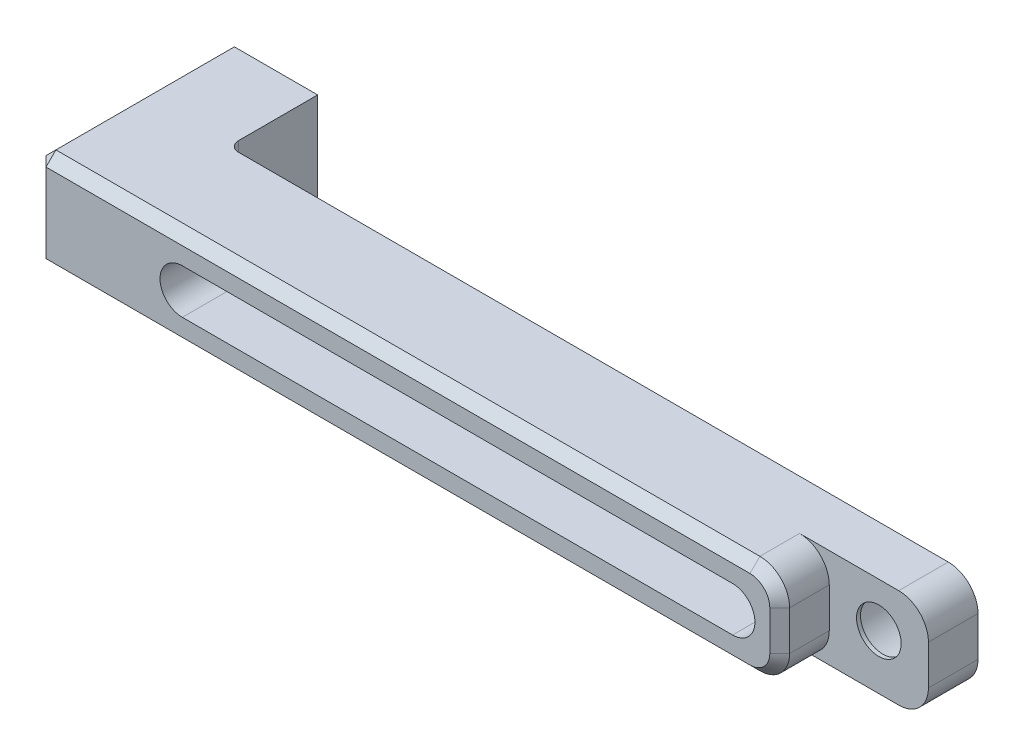
SolidWorks part; units mm, degrees
ref_plane "Front Plane" through (0, 0, 0) normal (0, 0, 1) x (1, 0, 0)
ref_plane "Top Plane" through (0, 0, 0) normal (0, 1, 0) x (1, 0, 0)
ref_plane "Right Plane" through (0, 0, 0) normal (1, 0, 0) x (0, 0, -1)
sketch "Sketch1" plane through (0, 0, 0) normal (0, 1, 0) x (1, 0, 0)
  line L1 (42.5, -5) -> (-42.5, -5)
  line L2 (42.5, -5) -> (42.5, 5)
  line L3 (42.5, 5) -> (-42.5, 5)
  line L4 (-42.5, -5) -> (-42.5, 5)
  line L5 (42.5, -5) -> (-42.5, 5) construction
  line L6 (42.5, 5) -> (-42.5, -5) construction
  point P0 (0, 0)
  dimension "D1" = 85
  dimension "D2" = 10
extrude "Boss-Extrude1" add sketch "Sketch1" along normal blind 10
sketch "Sketch2" plane through (0, 0, -5) normal (0, 0, 1) x (1, 0, 0)
  line L0 (0, 10) -> (0, 0) construction
  line L1 (-42.5, 10) -> (42.5, 10) construction
  line L2 (-27.75, 5) -> (27.75, 5) construction
  line L3 (-27.75, 9) -> (27.75, 9)
  line L4 (-27.75, 1) -> (27.75, 1)
  arc A0 (-27.75, 9) -> (-27.75, 1) centre (-27.75, 5) ccw
  arc A1 (27.75, 1) -> (27.75, 9) centre (27.75, 5) ccw
  point P7 (0, 5)
  dimension "D2" = 4
  dimension "D1" = 55.5
extrude "Cut-Extrude1" cut sketch "Sketch2" along normal blind 4.4
sketch "Sketch3" plane through (0, 0, -0.6) normal (0, 0, -1) x (-1, 0, 0)
  line L0 (-27.75, 5) -> (27.75, 5) construction
  line L1 (-27.75, 7.25) -> (27.75, 7.25)
  line L2 (-27.75, 2.75) -> (27.75, 2.75)
  line L3 (0, 0) -> (0, 10) construction
  line L4 (-42.5, 10) -> (42.5, 10) construction
  arc A0 (-27.75, 7.25) -> (-27.75, 2.75) centre (-27.75, 5) ccw
  arc A1 (27.75, 2.75) -> (27.75, 7.25) centre (27.75, 5) ccw
  point P4 (0, 5)
  dimension "D1" = 2.25
  dimension "D2" = 55.5
extrude "Cut-Extrude2" cut sketch "Sketch3" against normal through all
sketch "Sketch4" plane through (0, 0, -5) normal (0, 0, 1) x (1, 0, 0)
  line L0 (-42.5, 0) -> (42.5, 0) construction
  line L1 (-42.5, 10) -> (-33.1, 10)
  line L2 (-42.5, 10) -> (-42.5, 0)
  line L3 (-42.5, 0) -> (-33.1, 0)
  line L4 (-33.1, 10) -> (-33.1, 0)
  dimension "D1" = 9.4
extrude "Boss-Extrude2" add sketch "Sketch4" against normal blind 10 contours L4 L3 L2 L1
sketch "Sketch5" plane through (0, 0, 5) normal (0, 0, 1) x (1, 0, 0)
  line L0 (-42.5, 0) -> (42.5, 0) construction
  line L1 (42.5, 10) -> (32.5, 10)
  line L2 (42.5, 10) -> (42.5, 0)
  line L3 (42.5, 0) -> (32.5, 0)
  line L4 (32.5, 10) -> (32.5, 0)
  dimension "D1" = 10
extrude "Cut-Extrude3" cut sketch "Sketch5" against normal blind 5
sketch "Sketch6" plane through (0, 0, -15) normal (0, 0, -1) x (-1, 0, 0)
hole_wizard "M6 Tapped Hole1" positions "Sketch8" profile "Sketch9" tap size "M6" standard "GB"
sketch "Sketch8" plane through (0, 0, -15) normal (0, 0, -1) x (-1, 0, 0)
  point P0 (37.8, 4.8025)
sketch "Sketch9" plane through (-37.8, 4.8025, -15) normal (1, 0, 0) x (0, 1, 0)
  line L0 (0, 0) -> (0, 6.5022)
  line L1 (0, 6.5022) -> (2.5, 5)
  line L2 (2.5, 5) -> (2.5, 0)
  line L5 (2.5, 0) -> (0, 0)
  line L10 (0, 6.5022) -> (-2.5, 5) construction
  line L11 (0, -6.35) -> (0, 107.95) construction
  dimension "螺纹孔钻头直径" = 5
  dimension "螺纹孔钻头深度" = 5
  dimension "导头角度" = 118
cosmetic thread "HoleThreadLine1" parameters "D1"=12, "D2"=6
sketch "Sketch10" plane through (0, 0, -5) normal (0, 0, -1) x (-1, 0, 0)
hole_wizard "CBORE for M4 Hexagon socket head cap screws1" positions "Sketch12" profile "Sketch11" counterbore size "M4" standard "GB"
sketch "Sketch12" plane through (0, 0, -5) normal (0, 0, -1) x (-1, 0, 0)
  line L0 (-42.5, 10) -> (-42.5, 0) construction
  line L2 (-42.5, 10) -> (-32.5, 10) construction
  point P0 (-37.5, 5.5)
  dimension "D1" = 5
  dimension "D2" = 4.5
sketch "Sketch11" plane through (37.5, 5.5, -5) normal (1, 0, 0) x (0, 1, 0)
  line L0 (0, 0) -> (0, 15.3519)
  line L1 (0, 15.3519) -> (2.25, 14)
  line L2 (2.25, 14) -> (2.25, 4.6)
  line L3 (2.25, 4.6) -> (4, 4.6)
  line L4 (4, 4.6) -> (4, 0)
  line L5 (4, 0) -> (0, 0)
  line L10 (0, 15.3519) -> (-2.25, 14) construction
  line L11 (0, -6.35) -> (0, 107.95) construction
  dimension "孔直径" = 4.5
  dimension "孔深度" = 14
  dimension "柱形沉头孔直径" = 8
  dimension "柱形沉头孔深度" = 4.6
  dimension "导头角度" = 118
fillet "Fillet1" radius 3 4 edges at (42.5, 0, -2.5) (42.5, 10, -2.5) (32.5, 0, 2.5) (32.5, 10, 2.5)
fillet "Fillet2" radius 1 1 edges at (-33.1, 5, -5)
chamfer "Chamfer1" distance 1 angle 45 12 edges at (-6.5, 0, 5) (-42.5, 0, -5) (-42.5, 10, -5) (-6.5, 10, 5) (-42.5, 5, 5) (-37.8, 10, -15) (-42.5, 5, -15) (-37.8, 0, -15) (-33.1, 5, -15) (32.5, 5, 5) (31.6213, 9.1213, 5) (31.6213, 0.8787, 5)
equation "\"1\"= \"代号代号\""
equation "\"2\"= \"名称代号\""
